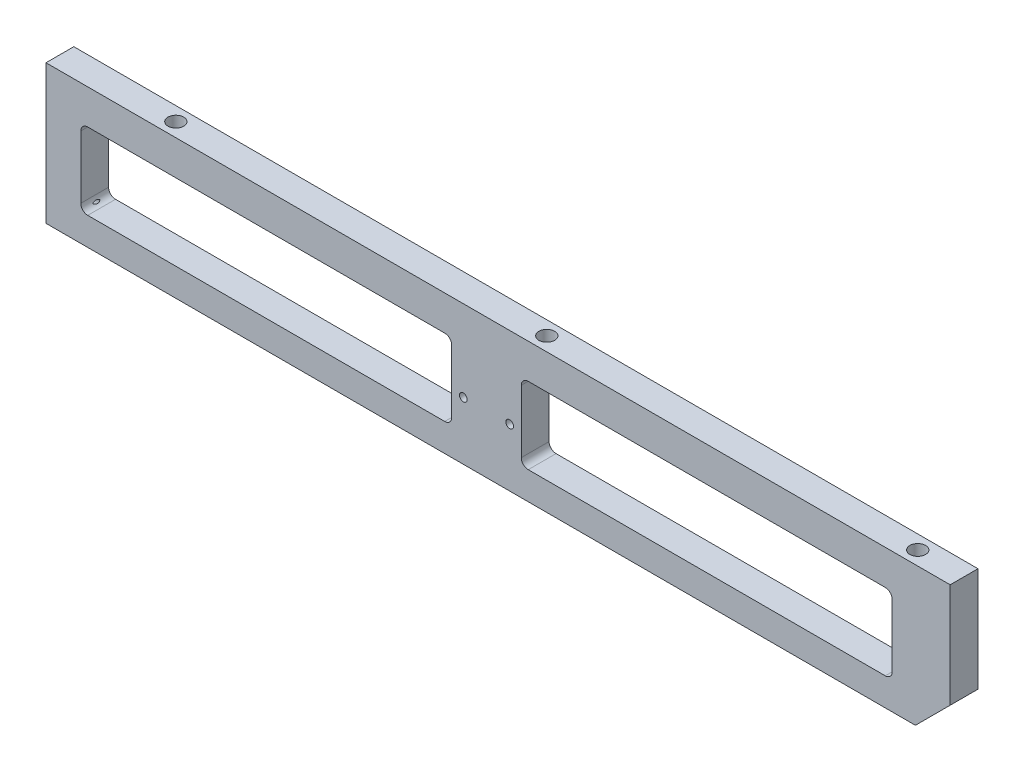
SolidWorks part; units mm, degrees
material "6061 合金"
ref_plane "前视基准面" through (0, 0, 0) normal (0, 0, 1) x (1, 0, 0)
ref_plane "上视基准面" through (0, 0, 0) normal (0, 1, 0) x (1, 0, 0)
ref_plane "右视基准面" through (0, 0, 0) normal (1, 0, 0) x (0, 0, -1)
sketch "草图1" plane through (0, 0, 0) normal (0, 0, 1) x (1, 0, 0)
  line L0 (180, -30) -> (195, -15)
  line L1 (180, -30) -> (-195, -30)
  line L2 (195, -15) -> (195, 30)
  line L3 (195, 30) -> (-195, 30)
  line L4 (-195, -30) -> (-195, 30)
  line L5 (195, -30) -> (-195, 30) construction
  line L6 (195, 30) -> (-195, -30) construction
  line L8 (-177, 15) -> (-23, 15)
  line L9 (-180, 12) -> (-180, -15)
  line L10 (-177, -18) -> (-23, -18)
  line L11 (-20, 12) -> (-20, -15)
  line L12 (13, 15) -> (167, 15)
  line L13 (10, 12) -> (10, -15)
  line L14 (13, -18) -> (167, -18)
  line L15 (170, 12) -> (170, -15)
  arc A0 (167, 15) -> (170, 12) centre (167, 12) cw
  arc A1 (170, -15) -> (167, -18) centre (167, -15) cw
  arc A2 (13, -18) -> (10, -15) centre (13, -15) cw
  arc A3 (10, 12) -> (13, 15) centre (13, 12) cw
  arc A4 (-23, 15) -> (-20, 12) centre (-23, 12) cw
  arc A5 (-20, -15) -> (-23, -18) centre (-23, -15) cw
  arc A6 (-180, -15) -> (-177, -18) centre (-177, -15) ccw
  arc A7 (-180, 12) -> (-177, 15) centre (-177, 12) cw
  point P0 (0, 0)
  dimension "D10" = 3
  dimension "D1" = 390
  dimension "D2" = 60
  dimension "D3" = 15
  dimension "D4" = 15
  dimension "D5" = 15
  dimension "D6" = 15
  dimension "D7" = 12
  dimension "D8" = 30
  dimension "D9" = 25
extrude "凸台-拉伸1" add sketch "草图1" along normal mid plane 12
hole_wizard "M8 螺纹孔1" positions "3D草图1" profile "草图3" tap size "M8" standard "GB"
sketch3d "3D草图1"
  line L4 (-195, 30, 6) -> (-195, -30, 6) construction
  line L5 (-195, 30, 6) -> (-195, 30, -6) construction
  line L6 (-195, -30, 6) -> (-195, -30, -6) construction
  point P0 (-195, 20, 0)
  point P2 (-195, -20, 0)
  dimension "D1" = 6
  dimension "D2" = 6
  dimension "D3" = 10
  dimension "D4" = 10
sketch "草图3" plane through (-195, 20, 0) normal (0, 1, 0) x (0, 0, 1)
  line L0 (0, 0) -> (0, 17.7929)
  line L1 (0, 17.7929) -> (3.4, 15.75)
  line L2 (3.4, 15.75) -> (3.4, 0)
  line L5 (3.4, 0) -> (0, 0)
  line L10 (0, 17.7929) -> (-3.4, 15.75) construction
  line L11 (0, -6.35) -> (0, 107.95) construction
  dimension "螺纹孔钻头直径" = 6.8
  dimension "螺纹孔钻头深度" = 15.75
  dimension "导头角度" = 118
cosmetic thread "孔螺蚊线4" parameters "D1"=12, "D2"=8
cosmetic thread "孔螺蚊线5" parameters "D1"=12, "D2"=8
hole_wizard "M4 螺纹孔1" positions "草图5" profile "草图4" tap size "M4" standard "GB" end condition through all
sketch "草图5" plane through (0, 0, 6) normal (0, 0, 1) x (1, 0, 0)
  line L0 (10, 12) -> (10, -15) construction
  line L1 (-195, -30) -> (180, -30) construction
  point P0 (-15, -5)
  point P2 (5, -5)
  dimension "D1" = 20
  dimension "D2" = 5
  dimension "D3" = 25
sketch "草图4" plane through (-15, -5, 6) normal (1, 0, 0) x (0, -1, 0)
  line L0 (0, 0) -> (0, 12)
  line L1 (0, 12) -> (1.65, 12)
  line L2 (1.65, 12) -> (1.65, 0)
  line L5 (1.65, 0) -> (0, 0)
  line L11 (0, -6.35) -> (0, 107.95) construction
  dimension "通孔螺纹孔钻头直径" = 3.3
  dimension "通孔螺纹孔钻头深度" = 12
cosmetic thread "孔螺蚊线6" parameters "D2"=4
cosmetic thread "孔螺蚊线7" parameters "D2"=4
hole_wizard "M8 螺纹孔2" positions "草图7" profile "草图6" tap size "M8" standard "GB"
sketch "草图7" plane through (0, 30, 0) normal (0, 1, 0) x (1, 0, 0)
  line L0 (-195, -6) -> (-195, 6) construction
  line L1 (195, 6) -> (-195, 6) construction
  point P0 (-145, 0)
  dimension "D1" = 50
  dimension "D2" = 6
sketch "草图6" plane through (-145, 30, 0) normal (1, 0, 0) x (0, 0, 1)
  line L0 (0, 0) -> (0, 17.7929)
  line L1 (0, 17.7929) -> (3.4, 15.75)
  line L2 (3.4, 15.75) -> (3.4, 0)
  line L5 (3.4, 0) -> (0, 0)
  line L10 (0, 17.7929) -> (-3.4, 15.75) construction
  line L11 (0, -6.35) -> (0, 107.95) construction
  dimension "螺纹孔钻头直径" = 6.8
  dimension "螺纹孔钻头深度" = 15.75
  dimension "导头角度" = 118
cosmetic thread "孔螺蚊线8" parameters "D1"=15, "D2"=8
pattern_linear "阵列(线性)1" count 3 spacing 160 along (1, 0, 0) of "M8 螺纹孔2"
